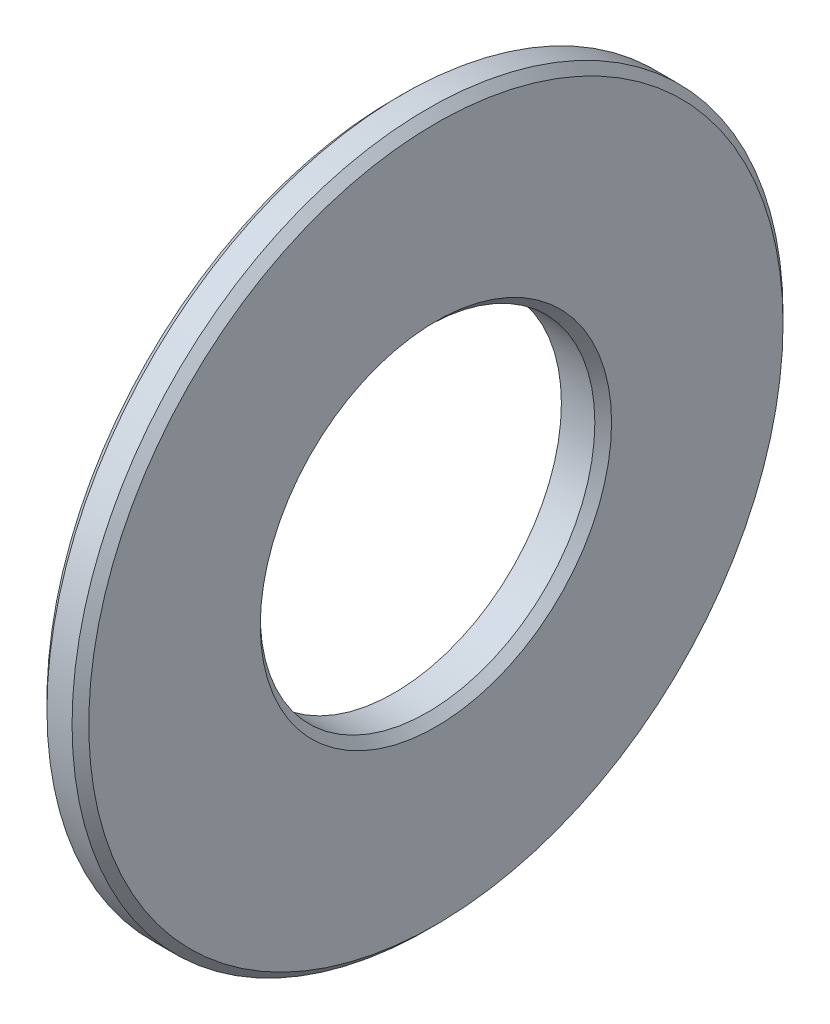
SolidWorks part; units mm, degrees
ref_plane "Front Plane" through (0, 0, 0) normal (0, 0, 1) x (1, 0, 0)
ref_plane "Top Plane" through (0, 0, 0) normal (0, 1, 0) x (1, 0, 0)
ref_plane "Right Plane" through (0, 0, 0) normal (1, 0, 0) x (0, 0, -1)
sketch "Sketch1" plane through (0, 0, 0) normal (1, 0, 0) x (0, 0, -1)
  circle A0 centre (0, 0) radius 40
  circle A1 centre (0, 0) radius 85
  dimension "D1" = 170
  dimension "D2" = 80
extrude "Boss-Extrude1" add sketch "Sketch1" along normal blind 10
chamfer "Chamfer1" distance 2 angle 45 3 edges at (0, 0, -85) (10, 0, -85) (10, 0, -40)
